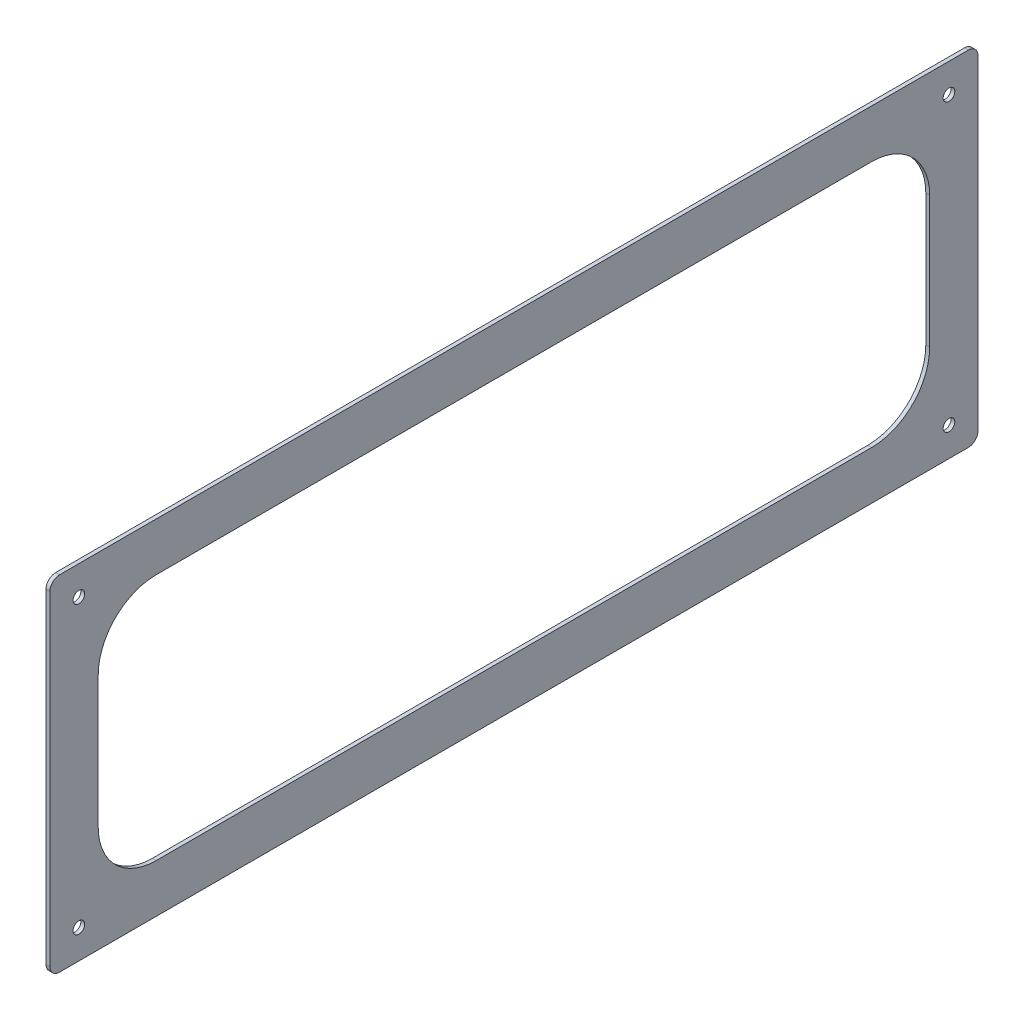
SolidWorks part; units mm, degrees
ref_plane "前视基准面" through (0, 0, 0) normal (0, 0, 1) x (1, 0, 0)
ref_plane "上视基准面" through (0, 0, 0) normal (0, 1, 0) x (1, 0, 0)
ref_plane "右视基准面" through (0, 0, 0) normal (1, 0, 0) x (0, 0, -1)
sketch "草图1" plane through (0, 0, 0) normal (1, 0, 0) x (0, 0, -1)
  line L0 (0, 89) -> (0, 0) construction
  line L1 (-240, 89) -> (240, 89)
  line L2 (-240, 89) -> (-240, -89)
  line L3 (-240, -89) -> (240, -89)
  line L4 (240, 89) -> (240, -89)
  line L5 (0, 0) -> (240, 0) construction
  dimension "D1" = 480
  dimension "D2" = 178
extrude "凸台-拉伸1" add sketch "草图1" along normal blind 2
sketch "草图2" plane through (2, 0, 0) normal (1, 0, 0) x (0, 0, -1)
  line L0 (0, 131.9543) -> (0, 0) construction
  line L1 (0, 0) -> (347.0268, 0) construction
  circle A0 centre (-225, 74) radius 3
  circle A1 centre (225, 74) radius 3
  circle A2 centre (-225, -74) radius 3
  circle A3 centre (225, -74) radius 3
  dimension "D1" = 6
  dimension "D2" = 450
  dimension "D3" = 148
extrude "切除-拉伸1" cut sketch "草图2" against normal through all
fillet "圆角1" radius 5 4 edges at (1, -89, 240) (1, -89, -240) (1, 89, -240) (1, 89, 240)
sketch "草图3" plane through (2, 0, 0) normal (1, 0, 0) x (0, 0, -1)
  line L0 (0, 234.3194) -> (0, 0) construction
  line L1 (-215, 64) -> (215, 64)
  line L2 (-215, 64) -> (-215, -64)
  line L3 (-215, -64) -> (215, -64)
  line L4 (215, 64) -> (215, -64)
  line L5 (0, 0) -> (371.0835, 0) construction
  dimension "D1" = 128
  dimension "D2" = 430
extrude "切除-拉伸2" cut sketch "草图3" against normal through all
fillet "圆角2" radius 30 4 edges at (1, -64, 215) (1, -64, -215) (1, 64, -215) (1, 64, 215)
